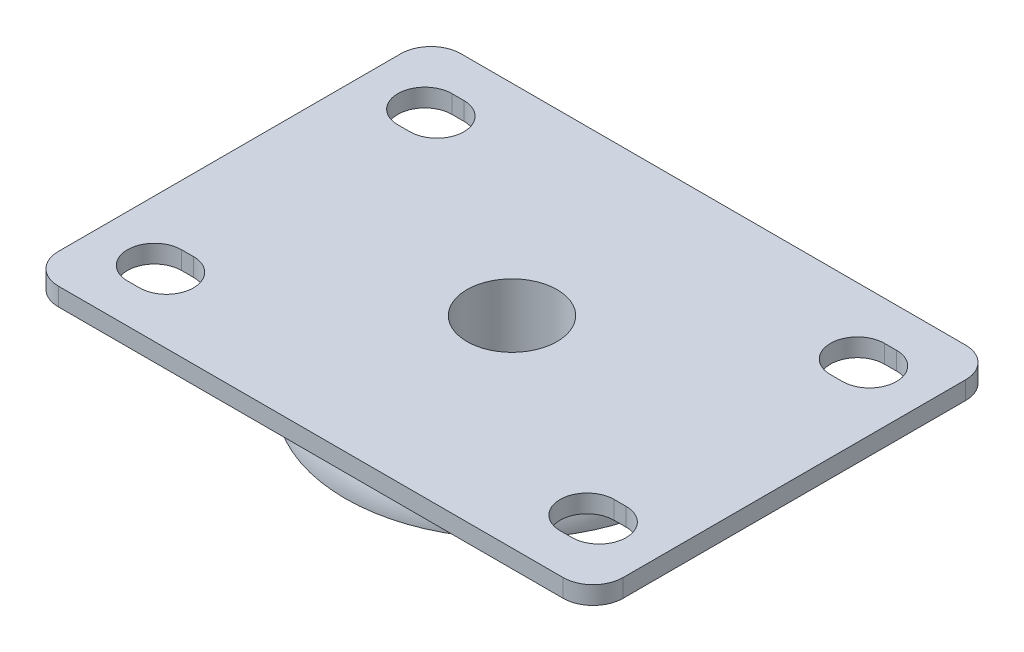
from build123d import *

# Parameters (mm, degrees)
SKETCH_2_W          = 94
SKETCH_2_H          = 67
EXTRUDE_1_DEPTH     = 3
FILLET_1_R          = 5
CUT_EXTRUDE_1_DEPTH = 58.794895968
SKETCH_6_R          = 7.5
CUT_EXTRUDE_2_DEPTH = 60.055059055


with BuildPart() as part:
    # 草图2 → 拉伸1 (new body)
    with BuildSketch(Plane(origin=(0, 0, 0), x_dir=(1, 0, 0), z_dir=(0, 1, 0))):
        Rectangle(SKETCH_2_W, SKETCH_2_H)
    extrude(amount=EXTRUDE_1_DEPTH)

    # 圆角1
    fillet_1_edges = [part.edges().sort_by_distance(p)[0] for p in [
        (-47, 1.5, -33.5),
        (47, 1.5, -33.5),
        (47, 1.5, 33.5),
        (-47, 1.5, 33.5),
    ]]
    fillet(fillet_1_edges, radius=FILLET_1_R)

    # 草图3 → 切除-拉伸1 (cut, through all)
    with BuildSketch(Plane(origin=(0, 3, 0), x_dir=(-1, 0, 0), z_dir=(0, 1, 0))):
        with BuildLine():
            Line((35, 27), (37, 27))
            ThreePointArc((37, 27), (41.5, 22.5), (37, 18))
            Line((37, 18), (35, 18))
            ThreePointArc((35, 18), (30.5, 22.5), (35, 27))
        make_face()
        with BuildLine():
            Line((-35, 18), (-37, 18))
            ThreePointArc((-37, 18), (-41.5, 22.5), (-37, 27))
            Line((-37, 27), (-35, 27))
            ThreePointArc((-35, 27), (-30.5, 22.5), (-35, 18))
        make_face()
        with BuildLine():
            Line((-35, -27), (-37, -27))
            ThreePointArc((-37, -27), (-41.5, -22.5), (-37, -18))
            Line((-37, -18), (-35, -18))
            ThreePointArc((-35, -18), (-30.5, -22.5), (-35, -27))
        make_face()
        with BuildLine():
            Line((35, -18), (37, -18))
            ThreePointArc((37, -18), (41.5, -22.5), (37, -27))
            Line((37, -27), (35, -27))
            ThreePointArc((35, -27), (30.5, -22.5), (35, -18))
        make_face()
    extrude(amount=-CUT_EXTRUDE_1_DEPTH, mode=Mode.SUBTRACT)

    # 草图4 → 旋转1 (revolve)
    with BuildSketch(Plane.XY, mode=Mode.PRIVATE) as revolve_1_sk:
        with BuildLine():
            Line((0, -9.5), (27.75, -9.5))
            ThreePointArc((27.75, -9.5), (24.967514421, -2.782485579), (18.25, 0))
            Line((18.25, 0), (0, 0))
            Line((0, 0), (0, -9.5))
        make_face()
    revolve(revolve_1_sk.sketch.rotate(Axis((0, 11.062770563, 0), (0, -1, 0)), 90), axis=Axis((0, 11.062770563, 0), (0, -1, 0)))

    # 草图6 → 切除-拉伸2 (cut, through all)
    with BuildSketch(Plane.XZ.offset(9.5)):
        with Locations(Location((0, 0, 0), (0, 0, 270))):
            Circle(SKETCH_6_R)
    extrude(amount=-CUT_EXTRUDE_2_DEPTH, mode=Mode.SUBTRACT)


solid = part.part
